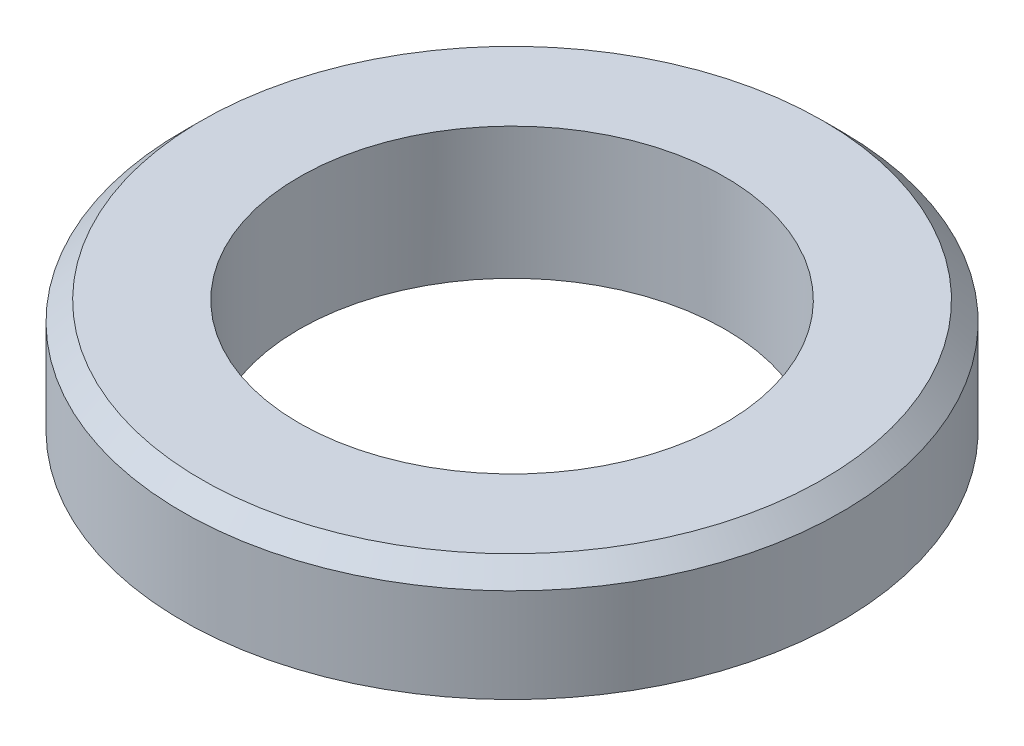
from build123d import *

# Parameters (mm, degrees)
G1_1_2_TAPPED_HOLE1_D     = 45.25
G1_1_2_TAPPED_HOLE1_DEPTH = 102.54
G1_1_2_TAPPED_HOLE1_TIP   = 13.594471505


with BuildPart() as part:
    # Sketch1 → Revolve1 (revolve)
    with BuildSketch(Plane(origin=(0, 0, 0), x_dir=(0, 0, -1), z_dir=(1, 0, 0))):
        Polygon((35, 12), (33, 14), (22.5, 14), (22.5, 0), (30, 0), (30, 2), (35, 2), align=None)
    revolve(axis=Axis((0, 0, 0), (0, 1, 0)))

    # G1-1/2 Tapped Hole1
    with Locations(Plane(origin=(0, 14, 0), x_dir=(1, 0, 0), z_dir=(0, 1, 0))):
        with Locations((0, 0)):
            Hole(G1_1_2_TAPPED_HOLE1_D / 2, depth=G1_1_2_TAPPED_HOLE1_DEPTH)
            with Locations((0, 0, -(G1_1_2_TAPPED_HOLE1_DEPTH + G1_1_2_TAPPED_HOLE1_TIP / 2))):  # 118° drill point
                Cone(0, G1_1_2_TAPPED_HOLE1_D / 2, G1_1_2_TAPPED_HOLE1_TIP, mode=Mode.SUBTRACT)


solid = part.part
